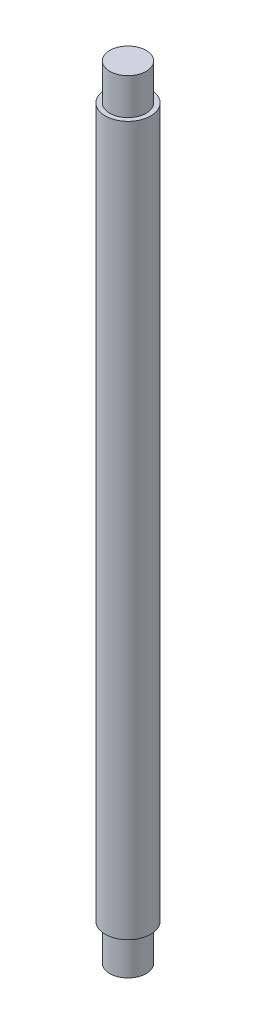
SolidWorks part; units mm, degrees
ref_plane "Front Plane" through (0, 0, 0) normal (0, 0, 1) x (1, 0, 0)
ref_plane "Top Plane" through (0, 0, 0) normal (0, 1, 0) x (1, 0, 0)
ref_plane "Right Plane" through (0, 0, 0) normal (1, 0, 0) x (0, 0, -1)
sketch "Sketch1" plane through (0, 0, 0) normal (0, 1, 0) x (1, 0, 0)
  circle A0 centre (0, 0) radius 5
  dimension "D1" = 10
extrude "Boss-Extrude1" add sketch "Sketch1" along normal mid plane 156
sketch "Sketch2" plane through (0, 78, 0) normal (0, 1, 0) x (1, 0, 0)
  circle A0 centre (0, 0) radius 4
  dimension "D1" = 8
extrude "Boss-Extrude2" add sketch "Sketch2" along normal blind 8
mirror "Mirror1" about plane through (0, 0, 0) normal (0, 1, 0) of "Boss-Extrude2"
